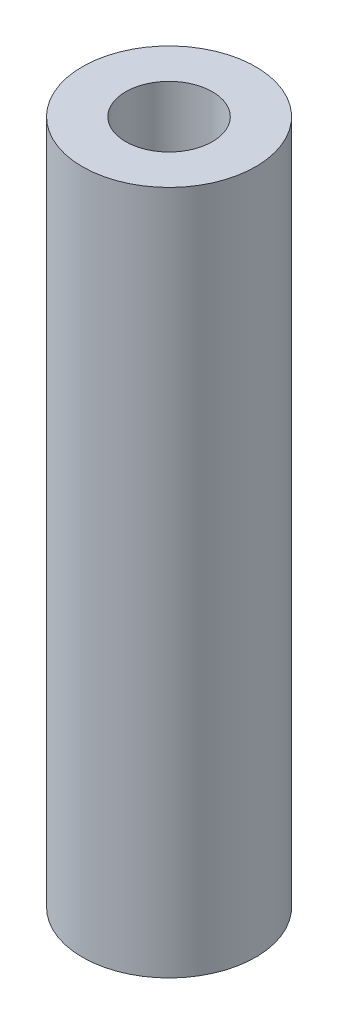
SolidWorks part; units mm, degrees
ref_plane "Front Plane" through (0, 0, 0) normal (0, 0, 1) x (1, 0, 0)
ref_plane "Top Plane" through (0, 0, 0) normal (0, 1, 0) x (1, 0, 0)
ref_plane "Right Plane" through (0, 0, 0) normal (1, 0, 0) x (0, 0, -1)
sketch "Sketch1" plane through (0, 0, 0) normal (0, 1, 0) x (1, 0, 0)
  circle A0 centre (0, 0) radius 5
  circle A1 centre (0, 0) radius 10
extrude "Boss-Extrude1" add sketch "Sketch1" along normal blind 79
